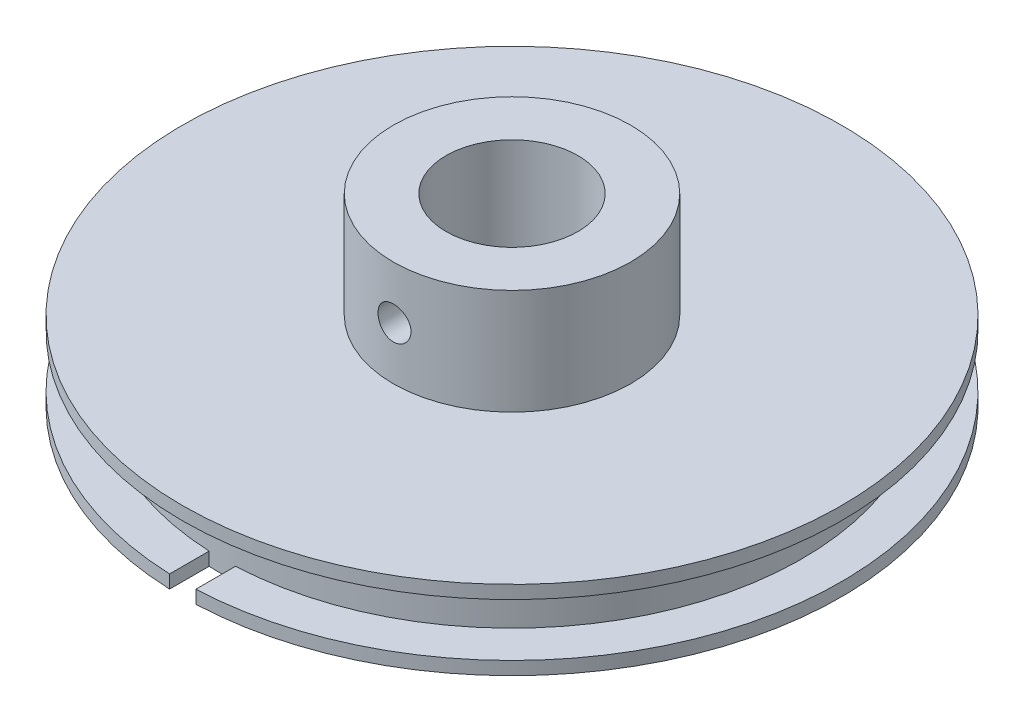
SolidWorks part; units mm, degrees
material "6061 合金"
ref_plane "Front Plane" through (0, 0, 0) normal (0, 0, 1) x (1, 0, 0)
ref_plane "Top Plane" through (0, 0, 0) normal (0, 1, 0) x (1, 0, 0)
ref_plane "Right Plane" through (0, 0, 0) normal (1, 0, 0) x (0, 0, -1)
sketch "Sketch1" plane through (0, 0, 0) normal (0, 0, 1) x (1, 0, 0)
  line L0 (0, 0) -> (0, -74.8686) construction
  line L1 (-5, 0) -> (-9, 0)
  line L2 (55, 0) -> (-55, 0) construction
  line L3 (-9, 0) -> (-9, -8)
  line L4 (-9, -8) -> (-25, -8)
  line L5 (-25, -8) -> (-25, -9)
  line L6 (-25, -14) -> (-5, -14)
  line L7 (-5, -14) -> (-5, 0)
  line L8 (-25, -9) -> (-22, -9)
  line L9 (-22, -9) -> (-22, -13)
  line L10 (-22, -13) -> (-25, -13)
  line L11 (-25, -13) -> (-25, -14)
  dimension "D1" = 5
  dimension "D2" = 22
  dimension "D3" = 25
  dimension "D4" = 6
  dimension "D5" = 1
  dimension "D6" = 1
  dimension "D7" = 14
  dimension "D8" = 9
revolve "Revolve1" add sketch "Sketch1" angle 360 about L0
sketch "Sketch2" plane through (0, -13, 0) normal (0, 1, 0) x (1, 0, 0)
  line L2 (-1, -21.9773) -> (-1, -40)
  line L3 (-1, -40) -> (1, -40)
  line L4 (1, -21.9773) -> (1, -40)
  circle A0 centre (0, 0) radius 22 construction
  arc A1 (-1, -21.9773) -> (1, -21.9773) centre (0, 0) ccw
  circle A2 centre (0, 0) radius 5 construction
  dimension "D1" = 1
  dimension "D2" = 2
  dimension "D3" = 40
extrude "Cut-Extrude1" cut sketch "Sketch2" against normal blind 10
ref_plane "Plane1" through (0, 0, 9) normal (0, 0, 1) x (1, 0, 0)
sketch "Sketch5" plane through (0, 0, 9) normal (0, 0, 1) x (1, 0, 0)
  point P0 (0, -4)
  dimension "D1" = 4
hole_wizard "M3 Tapped Hole1" positions "3DSketch2" profile "Sketch6" tap size "M3" standard "GB"
sketch3d "3DSketch2"
  point P3 (0, -4, 9)
sketch "Sketch6" plane through (0, -4, 9) normal (1, 0, 0) x (0, -1, 0)
  line L0 (0, 0) -> (0, 8.2511)
  line L1 (0, 8.2511) -> (1.25, 7.5)
  line L2 (1.25, 7.5) -> (1.25, 0)
  line L5 (1.25, 0) -> (0, 0)
  line L10 (0, 8.2511) -> (-1.25, 7.5) construction
  line L11 (0, -6.35) -> (0, 107.95) construction
  dimension "螺纹孔钻头直径" = 2.5
  dimension "螺纹孔钻头深度" = 7.5
  dimension "导头角度" = 118
